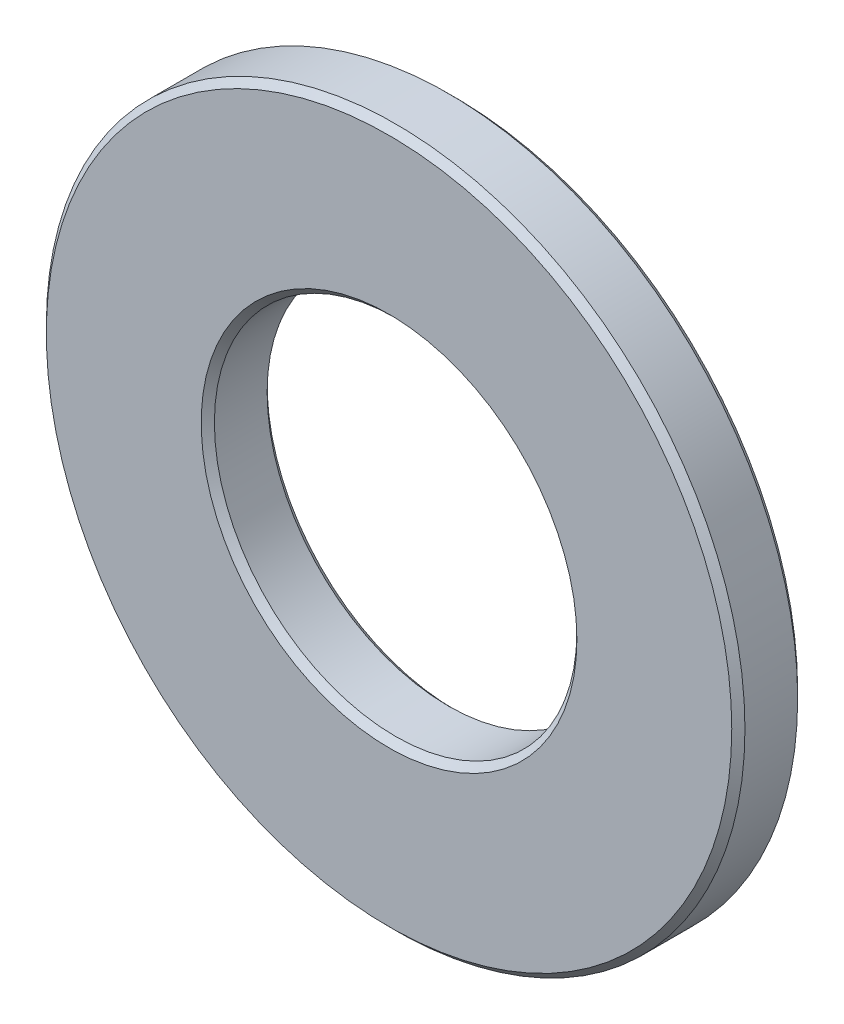
SolidWorks part; units mm, degrees
ref_plane "Front Plane" through (0, 0, 0) normal (0, 0, 1) x (1, 0, 0)
ref_plane "Top Plane" through (0, 0, 0) normal (0, 1, 0) x (1, 0, 0)
ref_plane "Right Plane" through (0, 0, 0) normal (1, 0, 0) x (0, 0, -1)
sketch "Sketch1" plane through (0, 0, 0) normal (0, 0, 1) x (1, 0, 0)
  circle A0 centre (0, 0) radius 27.5
  circle A1 centre (0, 0) radius 53
  dimension "D1" = 55
  dimension "D2" = 106
extrude "Boss-Extrude1" add sketch "Sketch1" along normal blind 10
chamfer "Chamfer1" distance 1 angle 45 4 edges at (53, 0, 0) (53, 0, 10) (27.5, 0, 0) (27.5, 0, 10)
